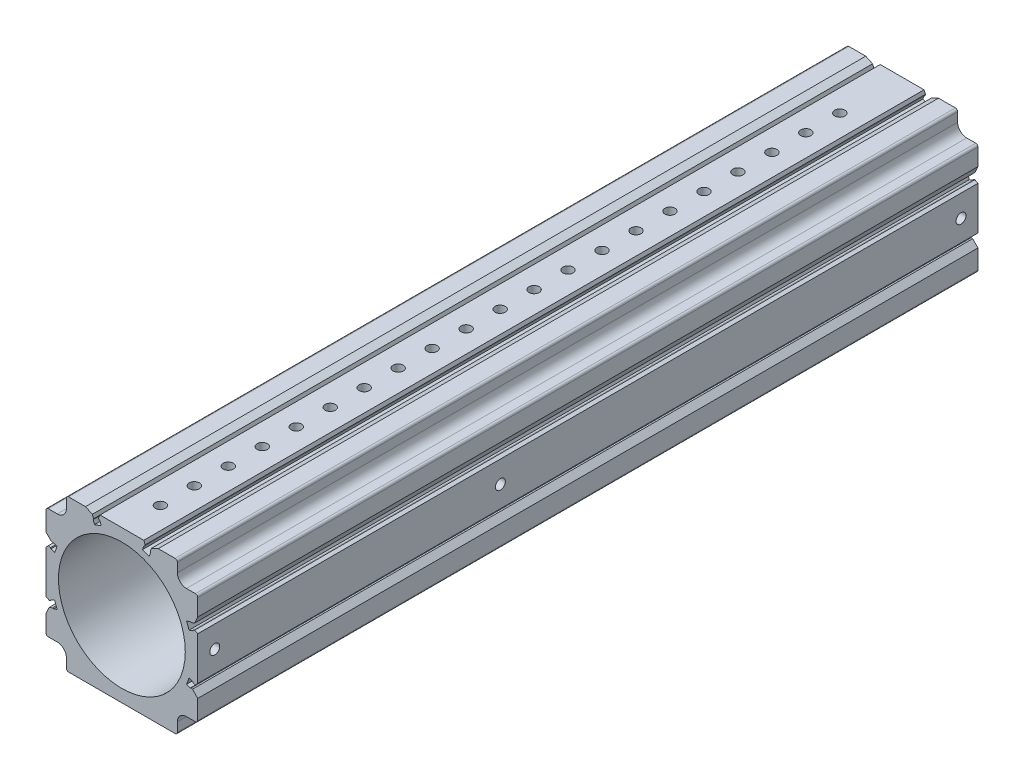
SolidWorks part; units mm, degrees
material "电镀钢"
ref_plane "Front Plane" through (0, 0, 0) normal (0, 0, 1) x (1, 0, 0)
ref_plane "Top Plane" through (0, 0, 0) normal (0, 1, 0) x (1, 0, 0)
ref_plane "Right Plane" through (0, 0, 0) normal (1, 0, 0) x (0, 0, -1)
sketch "Sketch1" plane through (0, 0, 0) normal (0, 0, 1) x (1, 0, 0)
  line L0 (-44.8, 67) -> (-36.9132, 67)
  line L1 (36.9132, 67) -> (44.8, 67)
  line L2 (67, 36.9132) -> (67, 44.8)
  line L3 (67, -44.8) -> (67, -36.9132)
  line L4 (-44.8, -67) -> (-36.9132, -67)
  line L5 (36.9132, -67) -> (44.8, -67)
  line L6 (-67, -44.8) -> (-67, -36.9132)
  line L7 (-67, 44.8) -> (-67, 36.9132)
  line L77 (67, -32.6) -> (67, -36.9132)
  line L79 (67, 27.5) -> (66.1, 27.5)
  line L80 (67, 57) -> (67, 44.8)
  line L81 (66.1, 32.6) -> (67, 32.6)
  line L82 (67, 27.5) -> (67, -27.5)
  line L83 (66.1, -27.5) -> (67, -27.5)
  line L84 (67, -32.6) -> (66.1, -32.6)
  line L85 (67, 36.9132) -> (67, 32.6)
  line L86 (65.5, -26.9) -> (62, -26.9)
  line L87 (62, 26.9) -> (65.5, 26.9)
  line L88 (62, -33.2) -> (65.5, -33.2)
  line L89 (65.5, 33.2) -> (62, 33.2)
  line L90 (62, -26.9) -> (62, -33.2)
  line L91 (62, 33.2) -> (62, 26.9)
  line L92 (57, -67) -> (44.8, -67)
  line L94 (67, -44.8) -> (67, -57)
  line L98 (44.8, 67) -> (57, 67)
  line L99 (32.6, 67) -> (36.9132, 67)
  line L100 (-36.9132, -67) -> (36.9132, -67)
  line L101 (33.2, 62) -> (33.2, 65.5)
  line L102 (26.9, 62) -> (33.2, 62)
  line L105 (32.6, 67) -> (32.6, 66.1)
  line L106 (27.5, 66.1) -> (27.5, 67)
  line L107 (-27.5, 67) -> (27.5, 67)
  line L108 (26.9, 65.5) -> (26.9, 62)
  line L109 (-33.2, 62) -> (-26.9, 62)
  line L110 (-26.9, 62) -> (-26.9, 65.5)
  line L111 (-27.5, 67) -> (-27.5, 66.1)
  line L112 (-36.9132, 67) -> (-32.6, 67)
  line L113 (-32.6, 66.1) -> (-32.6, 67)
  line L114 (-33.2, 65.5) -> (-33.2, 62)
  line L116 (-44.8, -67) -> (-57, -67)
  line L120 (-57, 67) -> (-44.8, 67)
  line L122 (-67, 32.6) -> (-67, 36.9132)
  line L123 (-62, 26.9) -> (-62, 33.2)
  line L124 (-65.5, 26.9) -> (-62, 26.9)
  line L125 (-62, 33.2) -> (-65.5, 33.2)
  line L126 (-62, -33.2) -> (-62, -26.9)
  line L127 (-62, -26.9) -> (-65.5, -26.9)
  line L128 (-65.5, -33.2) -> (-62, -33.2)
  line L130 (-67, 32.6) -> (-66.1, 32.6)
  line L131 (-67, -27.5) -> (-66.1, -27.5)
  line L132 (-66.1, 27.5) -> (-67, 27.5)
  line L133 (-66.1, -32.6) -> (-67, -32.6)
  line L134 (-67, -57) -> (-67, -44.8)
  line L135 (-67, -36.9132) -> (-67, -32.6)
  line L136 (-67, -27.5) -> (-67, 27.5)
  line L139 (-67, 44.8) -> (-67, 57)
  line L140 (-65.5, 33.2) -> (-66.1, 32.6)
  line L141 (-66.1, 27.5) -> (-65.5, 26.9)
  line L142 (-65.5, -26.9) -> (-66.1, -27.5)
  line L143 (-66.1, -32.6) -> (-65.5, -33.2)
  line L144 (65.5, -33.2) -> (66.1, -32.6)
  line L145 (66.1, -27.5) -> (65.5, -26.9)
  line L146 (65.5, 26.9) -> (66.1, 27.5)
  line L147 (66.1, 32.6) -> (65.5, 33.2)
  line L148 (33.2, 65.5) -> (32.6, 66.1)
  line L149 (27.5, 66.1) -> (26.9, 65.5)
  line L150 (-26.9, 65.5) -> (-27.5, 66.1)
  line L151 (-32.6, 66.1) -> (-33.2, 65.5)
  arc A15 (-67, -57) -> (-57, -67) centre (-57, -57) ccw
  arc A18 (57, -67) -> (67, -57) centre (57, -57) ccw
  arc A21 (67, 57) -> (57, 67) centre (57, 57) ccw
  arc A24 (-57, 67) -> (-67, 57) centre (-57, 57) ccw
  circle A25 centre (0, 0) radius 56
extrude "Boss-Extrude1" add sketch "Sketch1" along normal blind 689
sketch "Sketch3" plane through (0, 0, 689) normal (0, 0, 1) x (1, 0, 0)
  line L1 (-49, 49) -> (-73.0007, 49)
  line L2 (-49, 49) -> (-49, 80.3117)
  line L3 (-49, 80.3117) -> (-73.0007, 80.3117)
  line L4 (-73.0007, 49) -> (-73.0007, 80.3117)
  line L5 (-49, 49) -> (-73.0007, 80.3117) construction
  line L6 (-49, 80.3117) -> (-73.0007, 49) construction
  line L8 (-32.6, 67) -> (-57, 67) construction
  line L9 (-67, 57) -> (-67, 32.6) construction
  point P0 (-61.0004, 64.6558)
  dimension "D1" = 18
  dimension "D2" = 18
extrude "Cut-Extrude2" cut sketch "Sketch3" against normal through all
fillet "Fillet1" radius 8 1 edges at (-49, 49, 344.5)
pattern_circular "CirPattern1" count 4 over 360 about axis through (0, 0, 0) along (0, 0, 1) of "Cut-Extrude2", "Fillet1"
hole_wizard "Ø9.0 (9) Diameter Hole1" positions "Sketch6" profile "Sketch8" hole size "Ø9.0" standard "GB"
sketch "Sketch6" plane through (0, 67, 0) normal (0, -1, 0) x (-1, 0, 0)
  line L0 (0, 0) -> (0, -285.4047) construction
  line L4 (49, -689) -> (-49, -689) construction
  point P0 (0, -655)
  dimension "D1" = 34
sketch "Sketch8" plane through (0, 67, 655) normal (1, 0, 0) x (0, 0, 1)
  line L0 (0, 0) -> (0, 22.7039)
  line L1 (0, 22.7039) -> (4.5, 20)
  line L2 (4.5, 20) -> (4.5, 0)
  line L5 (4.5, 0) -> (0, 0)
  line L10 (0, 22.7039) -> (-4.5, 20) construction
  line L11 (0, -6.35) -> (0, 107.95) construction
  dimension "孔直径" = 9
  dimension "孔深度" = 20
  dimension "导头角度" = 118
hole_wizard "M12 Tapped Hole1" positions "Sketch9" profile "Sketch11" tap size "M12" standard "GB"
sketch "Sketch9" plane through (67, -134, 0) normal (-1, 0, 0) x (0, 0, -1)
  line L0 (0, -134) -> (-113.15, -134) construction
  line L4 (-411, -106.5) -> (-411, -161.5) construction
  point P2 (-394, -134)
  dimension "D1" = 17
sketch "Sketch11" plane through (67, 0, 394) normal (0, 1, 0) x (0, 0, -1)
  line L0 (0, 0) -> (0, 32.3144)
  line L1 (0, 32.3144) -> (5.1, 29.25)
  line L2 (5.1, 29.25) -> (5.1, 0)
  line L5 (5.1, 0) -> (0, 0)
  line L10 (0, 32.3144) -> (-5.1, 29.25) construction
  line L11 (0, -6.35) -> (0, 107.95) construction
  dimension "螺纹孔钻头直径" = 10.2
  dimension "螺纹孔钻头深度" = 29.25
  dimension "导头角度" = 118
cosmetic thread "Cosmetic Thread4" [suppressed] parameters "D1"=4.7084, "D2"=12
hole_wizard "M12 Tapped Hole2" positions "Sketch16" profile "Sketch17" tap size "M12" standard "GB"
sketch "Sketch16" plane through (67, 0, 0) normal (-1, 0, 0) x (0, 0, 1)
  point P0 (17, 0)
  dimension "D1" = 17
sketch "Sketch17" plane through (67, 0, 17) normal (0, 1, 0) x (0, 0, -1)
  line L0 (0, 0) -> (0, 32.3144)
  line L1 (0, 32.3144) -> (5.1, 29.25)
  line L2 (5.1, 29.25) -> (5.1, 0)
  line L5 (5.1, 0) -> (0, 0)
  line L10 (0, 32.3144) -> (-5.1, 29.25) construction
  line L11 (0, -6.35) -> (0, 107.95) construction
  dimension "螺纹孔钻头直径" = 10.2
  dimension "螺纹孔钻头深度" = 29.25
  dimension "导头角度" = 118
cosmetic thread "Cosmetic Thread5" [suppressed] parameters "D1"=4.7084, "D2"=12
pattern_linear "LPattern1" count 21 spacing 30 along (0, 0, -1) of "Ø9.0 (9) Diameter Hole1"
hole_wizard "G1/8 Tapped Hole1" positions "Sketch18" profile "Sketch19" tap size "G1/8" standard "GB"
sketch "Sketch18" plane through (67, 0, 0) normal (1, 0, 0) x (0, 0, -1)
  line L0 (-689, -27.5) -> (-689, 27.5) construction
  point P0 (-421.8, 0)
  dimension "D1" = 267.2
sketch "Sketch19" plane through (67, 0, 421.8) normal (0, 1, 0) x (0, 0, -1)
  line L0 (0, 0) -> (0, 24.8238)
  line L1 (0, 24.8238) -> (4.4, 22.18)
  line L2 (4.4, 22.18) -> (4.4, 0)
  line L5 (4.4, 0) -> (0, 0)
  line L10 (0, 24.8238) -> (-4.4, 22.18) construction
  line L11 (0, -6.35) -> (0, 107.95) construction
  dimension "螺纹孔钻头直径" = 8.8
  dimension "螺纹孔钻头深度" = 22.18
  dimension "导头角度" = 118
cosmetic thread "Cosmetic Thread9" parameters "D1"=4.6551, "D2"=9.728
fillet "Fillet2" radius 2 8 edges at (49, 67, 344.5) (67, 49, 344.5) (67, -49, 344.5) (49, -67, 344.5) (-49, -67, 344.5) (-67, -49, 344.5) (-67, 49, 344.5) (-49, 67, 344.5)
sketch "Sketch20" plane through (67, 0, 0) normal (1, 0, 0) x (0, 0, -1)
  line L0 (-674, 0) -> (-15, 0) construction
  line L1 (-689, -27.5) -> (-689, 27.5) construction
  line L2 (0, -27.5) -> (0, 27.5) construction
  circle A0 centre (-674, 0) radius 5
  circle A1 centre (-15, 0) radius 5
  dimension "D1" = 15
  dimension "D2" = 15
hole_wizard "G1/8 Tapped Hole2" positions "Sketch21" profile "Sketch22" tap size "G1/8" standard "GB"
sketch "Sketch21" plane through (67, 0, 0) normal (1, 0, 0) x (0, 0, -1)
  point P0 (-674, 0)
  point P3 (-15, 0)
sketch "Sketch22" plane through (67, 0, 674) normal (0, 1, 0) x (0, 0, -1)
  line L0 (0, 0) -> (0, 24.8238)
  line L1 (0, 24.8238) -> (4.4, 22.18)
  line L2 (4.4, 22.18) -> (4.4, 0)
  line L5 (4.4, 0) -> (0, 0)
  line L10 (0, 24.8238) -> (-4.4, 22.18) construction
  line L11 (0, -6.35) -> (0, 107.95) construction
  dimension "螺纹孔钻头直径" = 8.8
  dimension "螺纹孔钻头深度" = 22.18
  dimension "导头角度" = 118
cosmetic thread "Cosmetic Thread10" parameters "D1"=4.6551, "D2"=9.728
cosmetic thread "Cosmetic Thread11" parameters "D1"=4.6551, "D2"=9.728
sketch "Sketch23" plane through (0, 0, 0) normal (0, 0, -1) x (-1, 0, 0)
  line L0 (-23.1301, -51) -> (23.1301, -51)
  line L1 (47, -67) -> (-47, -67) construction
  circle A0 centre (0, 0) radius 56 construction
  arc A1 (-23.1301, -51) -> (23.1301, -51) centre (0, 0) ccw
  dimension "D1" = 16
extrude "Boss-Extrude2" [suppressed] add sketch "Sketch23" against normal through all
fillet "Fillet3" [suppressed] radius 10
other "Move Face1" [suppressed] parameters "D1"=6.5
sketch "Sketch24" plane through (0, 67, 0) normal (0, 1, 0) x (1, 0, 0)
  circle A0 centre (0, -655) radius 8
  dimension "D1" = 16
extrude "Cut-Extrude3" [suppressed] cut sketch "Sketch24" against normal blind 4
pattern_linear "LPattern2" [suppressed] count 7 spacing 30
sketch "Sketch25" plane through (0, 0, 689) normal (0, 0, 1) x (1, 0, 0)
  line L0 (0, 0) -> (0, 67) construction
  line L1 (27.5, 67) -> (-27.5, 67) construction
  line L2 (0, 0) -> (-25.07, 68.8793) construction
  line L3 (-18.2452, 59.3383) -> (-24.1653, 57.1836)
  line L4 (-24.1653, 57.1836) -> (-25.3624, 60.4725)
  line L5 (-18.2452, 59.3383) -> (-19.4423, 62.6272)
  line L6 (-25.3624, 60.4725) -> (-25.0037, 61.2415)
  line L7 (-25.0037, 61.2415) -> (-27.4907, 68.0745)
  line L8 (-19.4423, 62.6272) -> (-20.2113, 62.9858)
  line L9 (-20.2113, 62.9858) -> (-22.6983, 69.8188)
  line L10 (-22.6983, 69.8188) -> (-27.4907, 68.0745)
  circle A0 centre (0, 0) radius 56 construction
  dimension "D1" = 20
  dimension "D2" = 90
  dimension "D3" = 62
  dimension "D4" = 6.3
  dimension "D5" = 3.15
  dimension "D6" = 90
  dimension "D7" = 90
  dimension "D8" = 3.5
  dimension "D9" = 3.5
  dimension "D10" = 5.1
  dimension "D11" = 2.55
  dimension "D12" = 135
  dimension "D13" = 135
  dimension "D14" = 90
  dimension "D15" = 90
extrude "Cut-Extrude4" cut sketch "Sketch25" against normal through all
sketch "Sketch26" plane through (0, 0, 689) normal (0, 0, 1) x (1, 0, 0)
  line L0 (-27.5, 67) -> (-26.29, 64.4296)
  line L1 (-26.29, 64.4296) -> (-26.4603, 61.3407)
  line L2 (-26.4603, 61.3407) -> (-34.0001, 61.1462)
  line L3 (-34.0001, 61.1462) -> (-34.0001, 67)
  line L4 (-32.6, 67) -> (-47, 67) construction
  line L5 (-34.0001, 67) -> (-27.5, 67)
extrude "Boss-Extrude3" add sketch "Sketch26" against normal through all
chamfer "Chamfer2" distance 3 angle 45 1 edges at (-21.6724, 67, 344.5)
chamfer "Chamfer3" distance 3 angle 45 1 edges at (-27.0997, 67, 344.5)
mirror "Mirror1" about plane through (0, 0, 0) normal (1, 0, 0) of "Chamfer2", "Chamfer3", "Boss-Extrude3", "Cut-Extrude4"
pattern_circular "CirPattern13" count 4 over 360 about axis through (0, 0, 0) along (0, 0, 1) skipping 2 of "Cut-Extrude4"
pattern_circular "CirPattern14" count 4 over 360 about axis through (0, 0, 689) along (0, 0, -1) skipping 2 of "Boss-Extrude3"
mirror "Mirror2" about plane through (0, 0, 0) normal (0, 1, 0) of "CirPattern13", "Cut-Extrude4"
sketch "Sketch28" plane through (0, 0, 689) normal (0, 0, 1) x (1, 0, 0)
  line L0 (-27.0997, -67) -> (-21.6724, -67)
  line L1 (-21.6724, -67) -> (-15.1959, -57.9166)
  line L2 (-15.1959, -57.9166) -> (-28.9583, -52.9469)
  line L3 (-28.9583, -52.9469) -> (-27.0997, -67)
  line L4 (-67, 27.5) -> (-67, 32.6)
  line L5 (-67, 32.6) -> (-62.0056, 35.1671)
  line L6 (-62.0056, 35.1671) -> (-60.0646, 33.1648)
  line L7 (-60.0646, 33.1648) -> (-60.7664, 26.6143)
  line L8 (-60.7664, 26.6143) -> (-64.0283, 26.6143)
  line L9 (-64.0283, 26.6143) -> (-65.6774, 26.791)
  line L10 (-65.6774, 26.791) -> (-67, 27.5)
  line L11 (67, -27.5) -> (67, -32.6)
  line L12 (67, -32.6) -> (64.4183, -34.1929)
  line L13 (64.4183, -34.1929) -> (60.8641, -33.8121)
  line L14 (60.8641, -33.8121) -> (60.6405, -29.2349)
  line L15 (60.6405, -29.2349) -> (60.9192, -26.6336)
  line L16 (60.9192, -26.6336) -> (64.7514, -26.4463)
  line L17 (64.7514, -26.4463) -> (66.1689, -27.0788)
  line L18 (66.1689, -27.0788) -> (67, -27.5)
extrude "Boss-Extrude4" add sketch "Sketch28" against normal through all contours L3 L0 L1 L2 | L18 L11 L12 L13 L14 L15 L16 L17 | L10 L4 L5 L6 L7 L8 L9
chamfer "Chamfer4" distance 3 angle 45 8 edges at (-67, -21.6724, 344.5) (-67, -27.0997, 344.5) (67, 21.6724, 344.5) (67, 27.0997, 344.5) (-67, 27.0997, 344.5) (-67, 21.6724, 344.5) (67, -27.0997, 344.5) (67, -21.6724, 344.5)
